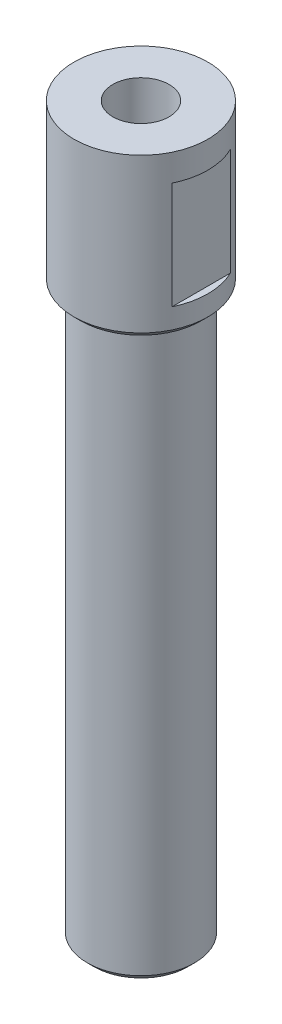
from build123d import *

# Parameters (mm, degrees)
SKETCH1_R             = 4
BOSS_EXTRUDE1_DEPTH   = 42.3
SKETCH2_R             = 5
BOSS_EXTRUDE2_DEPTH   = 12
M5_TAPPED_HOLE1_D     = 4.2
M5_TAPPED_HOLE1_DEPTH = 12.4
M5_TAPPED_HOLE1_TIP   = 1.2618073
M4_TAPPED_HOLE1_D     = 3.3
M4_TAPPED_HOLE1_DEPTH = 10.1
M4_TAPPED_HOLE1_TIP   = 0.991420021
SKETCH5_W             = 1
SKETCH5_H             = 8
CUT_EXTRUDE1_DEPTH    = 5
CHAMFER1_SIZE         = 0.5


with BuildPart() as part:
    # Sketch1 → Boss-Extrude1 (new body)
    with BuildSketch(Plane(origin=(0, 0, 0), x_dir=(1, 0, 0), z_dir=(0, 1, 0))):
        with Locations(Location((0, 0, 0), (0, 0, 270))):
            Circle(SKETCH1_R)
    extrude(amount=BOSS_EXTRUDE1_DEPTH)

    # Sketch2 → Boss-Extrude2 (add)
    with BuildSketch(Plane(origin=(0, 42.3, 0), x_dir=(1, 0, 0), z_dir=(0, 1, 0))):
        with Locations(Location((0, 0, 0), (0, 0, 270))):
            Circle(SKETCH2_R)
    extrude(amount=BOSS_EXTRUDE2_DEPTH)

    # M5 Tapped Hole1
    with Locations(Plane.ZX.offset(54.3)):
        with Locations((0, 0)):
            Hole(M5_TAPPED_HOLE1_D / 2, depth=M5_TAPPED_HOLE1_DEPTH)
            with Locations((0, 0, -(M5_TAPPED_HOLE1_DEPTH + M5_TAPPED_HOLE1_TIP / 2))):  # 118° drill point
                Cone(0, M5_TAPPED_HOLE1_D / 2, M5_TAPPED_HOLE1_TIP, mode=Mode.SUBTRACT)

    # M4 Tapped Hole1
    with Locations(Plane(origin=(0, 0, 0), x_dir=(0, 0, -1), z_dir=(0, -1, 0))):
        with Locations((0, 0)):
            Hole(M4_TAPPED_HOLE1_D / 2, depth=M4_TAPPED_HOLE1_DEPTH)
            with Locations((0, 0, -(M4_TAPPED_HOLE1_DEPTH + M4_TAPPED_HOLE1_TIP / 2))):  # 118° drill point
                Cone(0, M4_TAPPED_HOLE1_D / 2, M4_TAPPED_HOLE1_TIP, mode=Mode.SUBTRACT)

    # Sketch5 → Cut-Extrude1 (cut, symmetric)
    with BuildSketch(Plane.XY):
        with Locations((-5, 48.3)):
            Rectangle(SKETCH5_W, SKETCH5_H)
        with Locations((5, 48.3)):
            Rectangle(SKETCH5_W, SKETCH5_H)
    extrude(amount=CUT_EXTRUDE1_DEPTH, both=True, mode=Mode.SUBTRACT)

    # Chamfer1
    chamfer1_edges = [part.edges().sort_by_distance(p)[0] for p in [
        (0, 0, -4),
        (0, 42.3, -5),
    ]]
    chamfer(chamfer1_edges, length=CHAMFER1_SIZE)


solid = part.part
